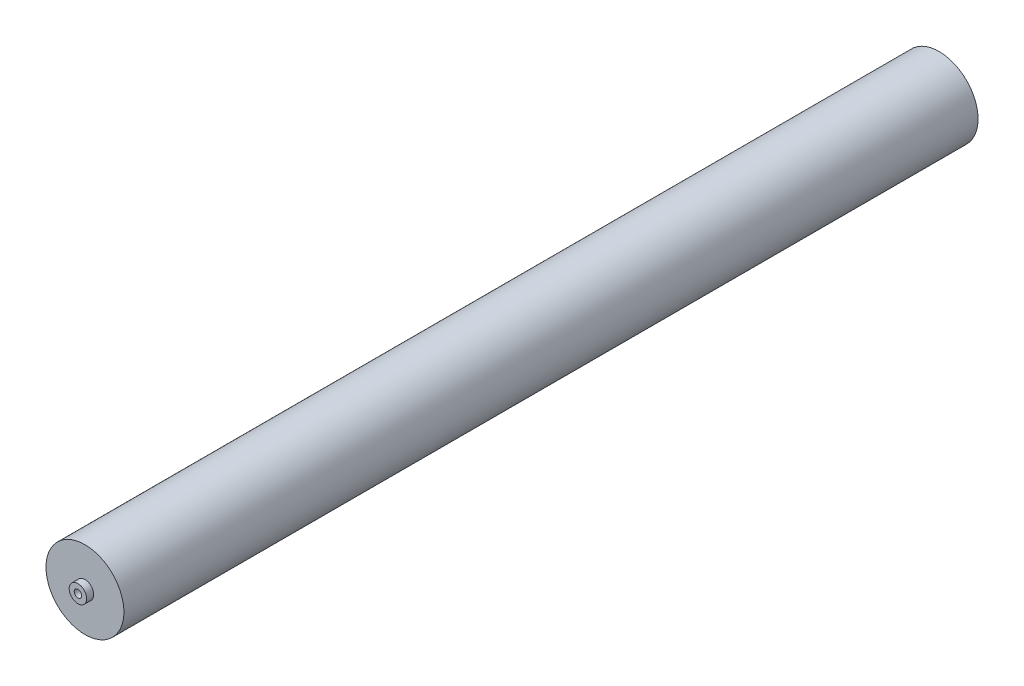
from build123d import *

# Parameters (mm, degrees)
SKETCH_1_R              = 44.5
EXTRUDE_1_DEPTH         = 976
SKETCH_2_R              = 10
EXTRUDE_2_DEPTH         = 8
EXTRUDE_START           = 8
SKETCH_3_R              = 10
EXTRUDE_3_DEPTH         = 8
HOLE_WIZARD_M10_1_D     = 8.5
HOLE_WIZARD_M10_1_DEPTH = 22.5
HOLE_WIZARD_M10_1_TIP   = 2.553657631
HOLE_WIZARD_M10_2_D     = 8.5
HOLE_WIZARD_M10_2_DEPTH = 22.5
HOLE_WIZARD_M10_2_TIP   = 2.553657631
SKETCH_11_R             = 7.5
CUT_EXTRUDE_1_DEPTH     = 488


with BuildPart() as part:
    # 草图1 → 凸台-拉伸1 (new body)
    with BuildSketch(Plane.XY):
        with Locations(Location((0, 0, 0), (0, 0, 180))):
            Circle(SKETCH_1_R)
    extrude(amount=EXTRUDE_1_DEPTH)

    # 草图2 → 凸台-拉伸2 (add)
    with BuildSketch(Plane.XY.offset(976)):
        Circle(SKETCH_2_R)
    extrude(amount=EXTRUDE_2_DEPTH)

    # 草图3 → 凸台-拉伸3 (add)
    with BuildSketch(Plane(origin=(0, 0, 0), x_dir=(-1, 0, 0), z_dir=(0, 0, -1)).offset(EXTRUDE_START)):
        with Locations(Location((0, 0, 0), (0, 0, 180))):
            Circle(SKETCH_3_R)
    extrude(amount=-EXTRUDE_3_DEPTH)

    # M10 螺纹孔1
    with Locations(Plane(origin=(0, 0, -8), x_dir=(-1, 0, 0), z_dir=(0, 0, -1))):
        with Locations((0, 0)):
            Hole(HOLE_WIZARD_M10_1_D / 2, depth=HOLE_WIZARD_M10_1_DEPTH)
            with Locations((0, 0, -(HOLE_WIZARD_M10_1_DEPTH + HOLE_WIZARD_M10_1_TIP / 2))):  # 118° drill point
                Cone(0, HOLE_WIZARD_M10_1_D / 2, HOLE_WIZARD_M10_1_TIP, mode=Mode.SUBTRACT)

    # M10 螺纹孔2
    with Locations(Plane.XY.offset(984)):
        with Locations((0, 0)):
            Hole(HOLE_WIZARD_M10_2_D / 2, depth=HOLE_WIZARD_M10_2_DEPTH)
            with Locations((0, 0, -(HOLE_WIZARD_M10_2_DEPTH + HOLE_WIZARD_M10_2_TIP / 2))):  # 118° drill point
                Cone(0, HOLE_WIZARD_M10_2_D / 2, HOLE_WIZARD_M10_2_TIP, mode=Mode.SUBTRACT)

    # 草图11 → 切除-拉伸1 (cut, symmetric)
    with BuildSketch(Plane.XY.offset(488)):
        Circle(SKETCH_11_R)
    extrude(amount=CUT_EXTRUDE_1_DEPTH, both=True, mode=Mode.SUBTRACT)


solid = part.part
